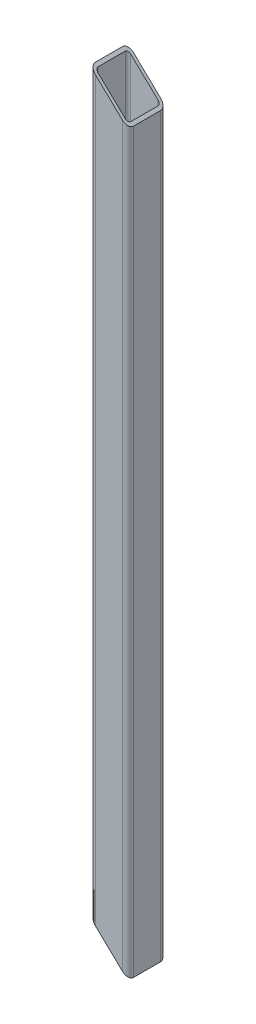
from build123d import *

# Parameters (mm, degrees)
F_19_WELDMEMBERFEAT_4_MORE_IN_5_FILES_DEPTH = 1420.5
CUT_EXTRUDE1_DEPTH                          = 1423.654297431
CUT_EXTRUDE1_DEPTH_BACK                     = 1423.654297431


with BuildPart() as part:
    # Sketch1 → 19 (WeldMemberFeat) (+4 more in 5 files) Cold-formed hollow square steel (GB/T 6728-2002) 70×70×5(1) (new body)
    with BuildSketch(Plane(origin=(0, 0, 0), x_dir=(-1, 0, 0), z_dir=(0, 1, 0))):
        with BuildLine():
            Line((-25, -35), (25, -35))
            ThreePointArc((25, -35), (32.071067812, -32.071067812), (35, -25))
            Line((35, -25), (35, 25))
            ThreePointArc((35, 25), (32.071067812, 32.071067812), (25, 35))
            Line((25, 35), (-25, 35))
            ThreePointArc((-25, 35), (-32.071067812, 32.071067812), (-35, 25))
            Line((-35, 25), (-35, -25))
            ThreePointArc((-35, -25), (-32.071067812, -32.071067812), (-25, -35))
        make_face()
        with BuildLine():
            Line((-25, -30), (25, -30))
            ThreePointArc((25, -30), (28.535533906, -28.535533906), (30, -25))
            Line((30, -25), (30, 25))
            ThreePointArc((30, 25), (28.535533906, 28.535533906), (25, 30))
            Line((25, 30), (-25, 30))
            ThreePointArc((-25, 30), (-28.535533906, 28.535533906), (-30, 25))
            Line((-30, 25), (-30, -25))
            ThreePointArc((-30, -25), (-28.535533906, -28.535533906), (-25, -30))
        make_face(mode=Mode.SUBTRACT)
    extrude(amount=F_19_WELDMEMBERFEAT_4_MORE_IN_5_FILES_DEPTH)

    # Sketch2 → Cut-Extrude1 (cut, two sides: drawn at the far end of the back side and taken through both)
    with BuildSketch(Plane.XY.offset(35).offset(-CUT_EXTRUDE1_DEPTH_BACK)):
        Polygon((-35, 66.713584391), (35, 0), (-35, 0), align=None)
        Polygon((-35, 1420.5), (35, 1353.786415609), (35, 1420.5), align=None)
    extrude(amount=CUT_EXTRUDE1_DEPTH + CUT_EXTRUDE1_DEPTH_BACK, mode=Mode.SUBTRACT)


solid = part.part
